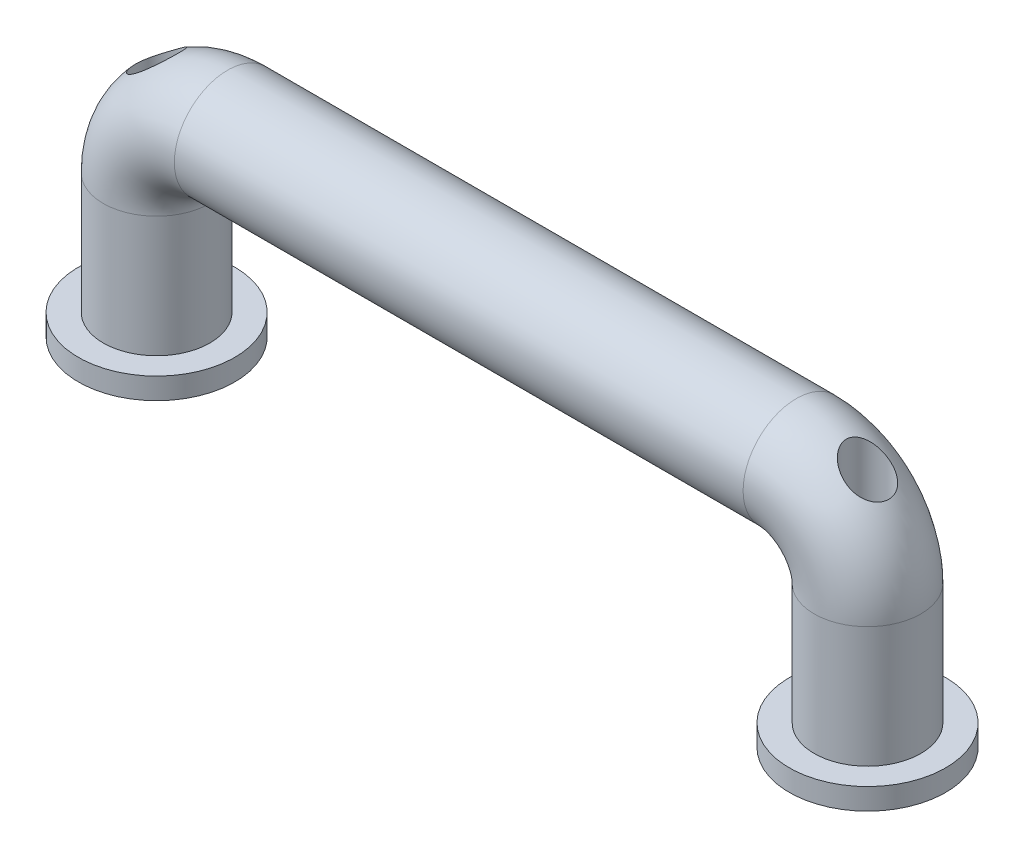
from build123d import *

# Parameters (mm, degrees)
SKETCH_2_R          = 7.5
SKETCH_3_R          = 11
EXTRUDE_1_DEPTH     = 3
SKETCH_4_R          = 1.65
CUT_EXTRUDE_1_DEPTH = 51
CUT_EXTRUDE_START   = -20
SKETCH_5_R          = 3
CUT_EXTRUDE_2_DEPTH = 51


with BuildPart() as part:
    # 扫描1: sweep along a path in 草图1
    with BuildLine(Plane.XY) as sweep_1_path:
        Line((0, 0), (0, 20))
        ThreePointArc((0, 20), (2.928932188, 27.071067812), (10, 30))
        Line((10, 30), (90, 30))
        ThreePointArc((90, 30), (97.071067812, 27.071067812), (100, 20))
        Line((100, 20), (100, 0))
    # 草图2 → 扫描1 (sweep)
    with BuildSketch(Plane(origin=(0, 0, 0), x_dir=(1, 0, 0), z_dir=(0, 1, 0))):
        Circle(SKETCH_2_R)
    sweep(path=sweep_1_path.line)

    # 草图3 → 凸台-拉伸1 (add)
    with BuildSketch(Plane.XZ):
        with Locations(Location((0, 0, 0), (0, 0, 270))):
            Circle(SKETCH_3_R)
        with Locations(Location((100, 0, 0), (0, 0, 270))):
            Circle(SKETCH_3_R)
    extrude(amount=-EXTRUDE_1_DEPTH)

    # 草图4 → 切除-拉伸1 (cut)
    with BuildSketch(Plane.XZ):
        with Locations(Location((0, 0, 0), (0, 0, 270))):
            Circle(SKETCH_4_R)
        with Locations(Location((100, 0, 0), (0, 0, 270))):
            Circle(SKETCH_4_R)
    extrude(amount=-CUT_EXTRUDE_1_DEPTH, mode=Mode.SUBTRACT)

    # 草图5 → 切除-拉伸2 (cut)
    with BuildSketch(Plane.XZ.offset(CUT_EXTRUDE_START)):
        with Locations(Location((0, 0, 0), (0, 0, 270))):
            Circle(SKETCH_5_R)
        with Locations(Location((100, 0, 0), (0, 0, 270))):
            Circle(SKETCH_5_R)
    extrude(amount=-CUT_EXTRUDE_2_DEPTH, mode=Mode.SUBTRACT)


solid = part.part
